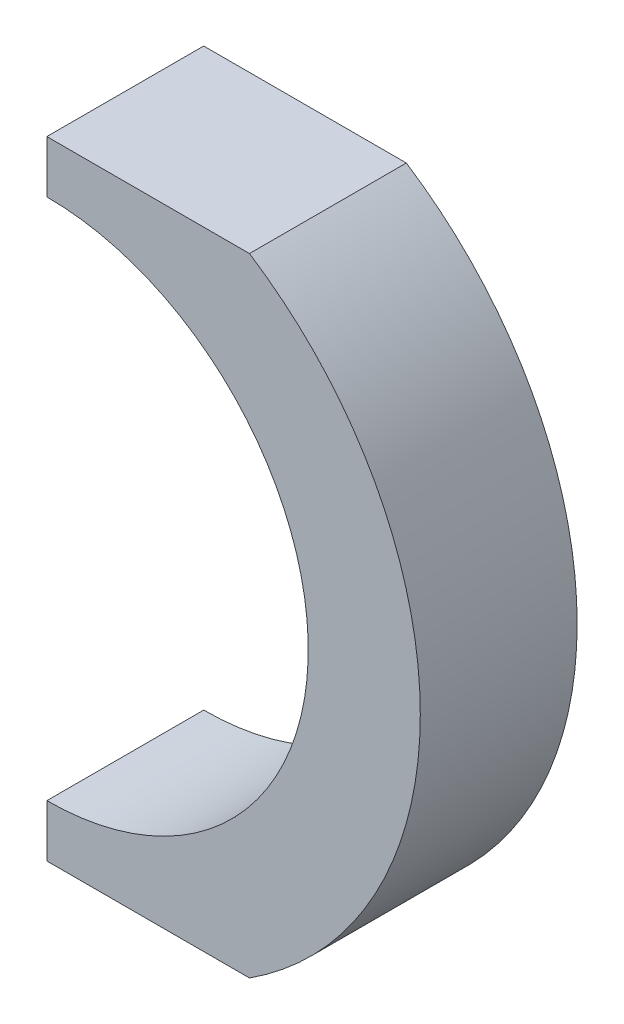
from build123d import *

# Parameters (mm, degrees)
SKETCH_1_R          = 100
EXTRUDE_1_DEPTH     = 42
CUT_EXTRUDE_1_DEPTH = 148.526268847
CUT_EXTRUDE_2_DEPTH = 138.186005117


with BuildPart() as part:
    # 草图1 → 凸台-拉伸1 (new body)
    with BuildSketch(Plane.XY):
        with Locations(Location((0, 0, 0), (0, 0, 180))):
            Circle(SKETCH_1_R)
    extrude(amount=EXTRUDE_1_DEPTH)

    # 草图2 → 切除-拉伸1 (cut, through all)
    with BuildSketch(Plane.XY.offset(42)):
        with BuildLine():
            Line((-54.258639865, 84), (54.258639865, 84))
            ThreePointArc((54.258639865, 84), (0, 100), (-54.258639865, 84))
        make_face()
        with BuildLine():
            Line((-54.258639865, -84), (54.258639865, -84))
            ThreePointArc((54.258639865, -84), (0, -100), (-54.258639865, -84))
        make_face()
    extrude(amount=-CUT_EXTRUDE_1_DEPTH, mode=Mode.SUBTRACT)

    # 草图3 → 切除-拉伸2 (cut, through all)
    with BuildSketch(Plane.XY.offset(42)):
        with BuildLine():
            Line((0, 70), (0, 84))
            Line((0, 84), (-54.258639865, 84))
            ThreePointArc((-54.258639865, 84), (-100, 0), (-54.258639865, -84))
            Line((-54.258639865, -84), (0, -84))
            Line((0, -84), (0, -70))
            ThreePointArc((0, -70), (70, 0), (0, 70))
        make_face()
    extrude(amount=-CUT_EXTRUDE_2_DEPTH, mode=Mode.SUBTRACT)


solid = part.part
